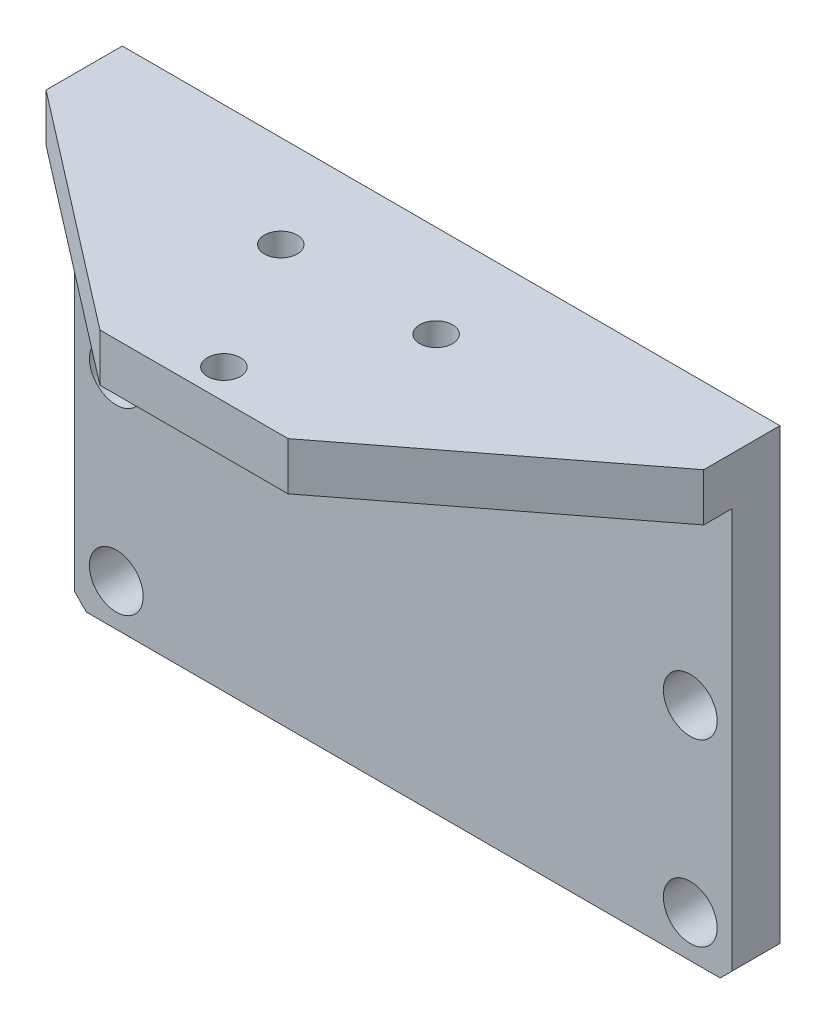
SolidWorks part; units mm, degrees
ref_plane "前视基准面" through (0, 0, 0) normal (0, 0, 1) x (1, 0, 0)
ref_plane "上视基准面" through (0, 0, 0) normal (0, 1, 0) x (1, 0, 0)
ref_plane "右视基准面" through (0, 0, 0) normal (1, 0, 0) x (0, 0, -1)
sketch "草图1" plane through (0, 0, 0) normal (0, 0, 1) x (1, 0, 0)
  line L1 (-55, 38.5) -> (55, 38.5)
  line L2 (-55, 38.5) -> (-55, -38.5)
  line L3 (-55, -38.5) -> (55, -38.5)
  line L4 (55, 38.5) -> (55, -38.5)
  line L5 (-55, 38.5) -> (55, -38.5) construction
  line L6 (-55, -38.5) -> (55, 38.5) construction
  point P0 (0, 0)
  dimension "D1" = 110
  dimension "D2" = 77
extrude "凸台-拉伸1" add sketch "草图1" along normal blind 8
sketch "草图2" plane through (0, 0, 0) normal (0, 0, 1) x (1, 0, 0)
  line L0 (55, -38.5) -> (55, 38.5) construction
  line L1 (-55, 38.5) -> (55, 38.5)
  line L2 (-55, 38.5) -> (-55, 30.5)
  line L3 (-55, 30.5) -> (55, 30.5)
  line L4 (55, 38.5) -> (55, 30.5)
  dimension "D1" = 8
extrude "凸台-拉伸3" add sketch "草图2" along normal blind 43 contours L3 L4 L1 L2
sketch "草图4" plane through (0, 38.5, 0) normal (0, 1, 0) x (1, 0, 0)
  line L0 (-55, -43) -> (55, -43) construction
  line L1 (-55, 0) -> (55, 0)
  line L2 (-55, 0) -> (-55, -12.75)
  line L3 (55, -43) -> (55, 0) construction
  line L4 (55, 0) -> (55, -12.75)
  line L5 (-15.74, -43) -> (15.74, -43)
  line L9 (-55, -12.75) -> (-15.74, -43)
  line L10 (15.74, -43) -> (55, -12.75)
  dimension "D1" = 12.75
  dimension "D2" = 31.48
  dimension "D3" = 15.74
  dimension "D4" = 12.75
extrude "切除-拉伸1" cut sketch "草图4" against normal blind 43 flip side to cut
hole_wizard "Ø7.0 (7) 直径孔1" positions "草图6" profile "草图5" hole size "Ø7.0" standard "ISO" end condition through all
sketch "草图6" plane through (0, 0, 8) normal (0, 0, 1) x (1, 0, 0)
  line L0 (-55, -38.5) -> (55, -38.5) construction
  point P0 (-48, -31.5)
  point P2 (48, -31.5)
  point P4 (48, -1.5)
  point P6 (-48, -1.5)
  dimension "D1" = 96
  dimension "D2" = 48
  dimension "D3" = 7
  dimension "D4" = 30
sketch "草图5" plane through (-48, -31.5, 8) normal (1, 0, 0) x (0, -1, 0)
  line L0 (0, 0) -> (0, 8)
  line L1 (0, 8) -> (4.5, 8)
  line L2 (4.5, 8) -> (4.5, 0)
  line L5 (4.5, 0) -> (0, 0)
  line L11 (0, -6.35) -> (0, 107.95) construction
  dimension "通孔孔直径" = 9
  dimension "通孔孔深度" = 8
hole_wizard "Ø5.5 (5.5) 直径孔2" positions "草图10" profile "草图9" hole size "Ø5.5" standard "ISO" end condition through all
sketch "草图10" plane through (0, 38.5, 0) normal (0, 1, 0) x (1, 0, 0)
  line L0 (-15.74, -43) -> (15.74, -43) construction
  line L2 (0, -43) -> (0, -17.2173) construction
  line L4 (0, -23) -> (25.9808, -8) construction
  line L6 (0, -23) -> (-29.592, -5.9151) construction
  circle A0 centre (0, -23) radius 15 construction
  point P0 (-12.9904, -15.5)
  point P2 (12.9904, -15.5)
  point P4 (0, -38)
  dimension "D1" = 30
  dimension "D2" = 120
  dimension "D3" = 120
  dimension "D6" = 20
sketch "草图9" plane through (-12.9904, 38.5, 15.5) normal (1, 0, 0) x (0, 0, 1)
  line L0 (0, 0) -> (0, 77)
  line L1 (0, 77) -> (2.75, 77)
  line L2 (2.75, 77) -> (2.75, 0)
  line L5 (2.75, 0) -> (0, 0)
  line L11 (0, -6.35) -> (0, 107.95) construction
  dimension "通孔孔直径" = 5.5
  dimension "通孔孔深度" = 77
chamfer "倒角1" distance 2 angle 45 2 edges at (-55, -38.5, 4) (55, -38.5, 4)
